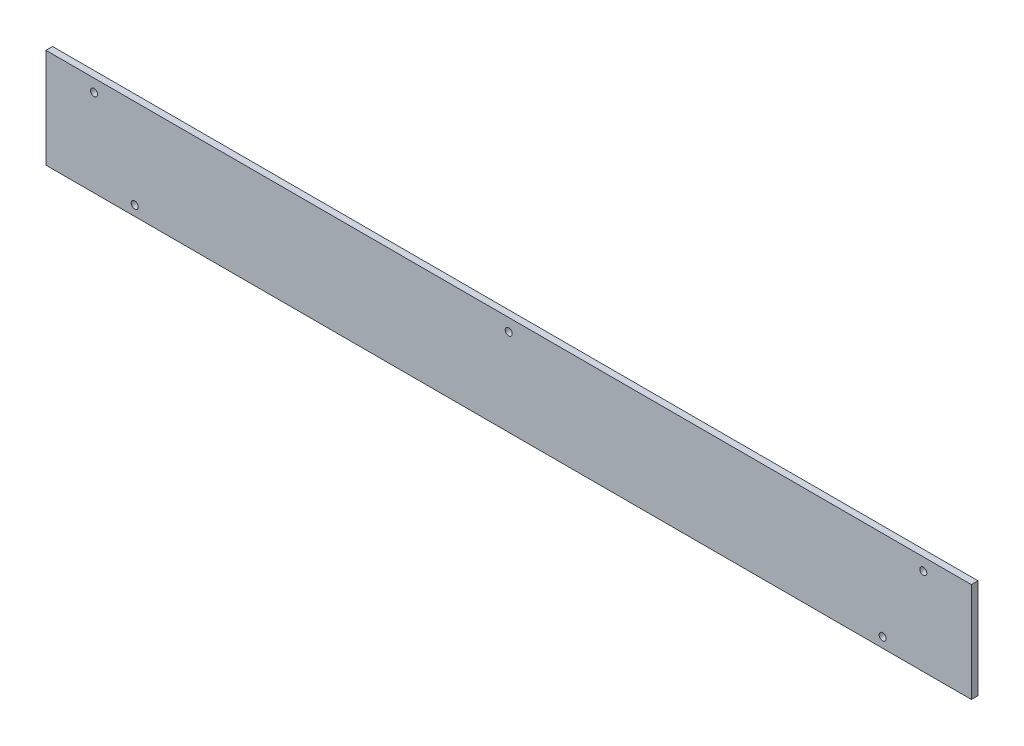
SolidWorks part; units mm, degrees
material "1023 碳钢板 (SS)"
ref_plane "Front Plane" through (0, 0, 0) normal (0, 0, 1) x (1, 0, 0)
ref_plane "Top Plane" through (0, 0, 0) normal (0, 1, 0) x (1, 0, 0)
ref_plane "Right Plane" through (0, 0, 0) normal (1, 0, 0) x (0, 0, -1)
sketch "Sketch1" plane through (0, 0, 0) normal (0, 0, 1) x (1, 0, 0)
  line L1 (-558, 60) -> (558, 60)
  line L2 (-558, 60) -> (-558, -60)
  line L3 (-558, -60) -> (558, -60)
  line L4 (558, 60) -> (558, -60)
  line L5 (-558, 60) -> (558, -60) construction
  line L6 (-558, -60) -> (558, 60) construction
  point P0 (0, 0)
  dimension "D1" = 1116
  dimension "D2" = 120
extrude "Boss-Extrude1" add sketch "Sketch1" along normal blind 8
sketch "Sketch2" plane through (0, 0, 8) normal (0, 0, 1) x (1, 0, 0)
  line L0 (558, -60) -> (558, 60) construction
  line L1 (558, 60) -> (-558, 60) construction
  line L2 (-558, 60) -> (-558, -60) construction
  circle A0 centre (-500, 45) radius 4
  circle A1 centre (0, 45) radius 4
  circle A2 centre (500, 45) radius 4
  circle A3 centre (-451, -48) radius 4
  circle A4 centre (451, -48) radius 4
  dimension "D8" = 8
  dimension "D1" = 1000
  dimension "D2" = 500
  dimension "D3" = 58
  dimension "D4" = 93
  dimension "D5" = 15
  dimension "D6" = 107
  dimension "D7" = 107
hole_wizard "M10 Tapped Hole1" positions "Sketch3" profile "Sketch4" tap size "M10" standard "ISO"
sketch "Sketch3" plane through (0, 0, 8) normal (0, 0, 1) x (1, 0, 0)
  point P0 (-500, 45)
  point P3 (-451, -48)
  point P6 (0, 45)
  point P9 (500, 45)
  point P12 (451, -48)
sketch "Sketch4" plane through (-500, 45, 8) normal (1, 0, 0) x (0, -1, 0)
  line L0 (0, 0) -> (0, 27.0537)
  line L1 (0, 27.0537) -> (4.25, 24.5)
  line L2 (4.25, 24.5) -> (4.25, 0)
  line L5 (4.25, 0) -> (0, 0)
  line L10 (0, 27.0537) -> (-4.25, 24.5) construction
  line L11 (0, -6.35) -> (0, 107.95) construction
  dimension "螺纹孔钻头直径" = 8.5
  dimension "螺纹孔钻头深度" = 24.5
  dimension "导头角度" = 118
cosmetic thread "Hole Thread Line1"
cosmetic thread "Hole Thread Line2"
cosmetic thread "Hole Thread Line3"
cosmetic thread "Hole Thread Line4"
cosmetic thread "Hole Thread Line5"
